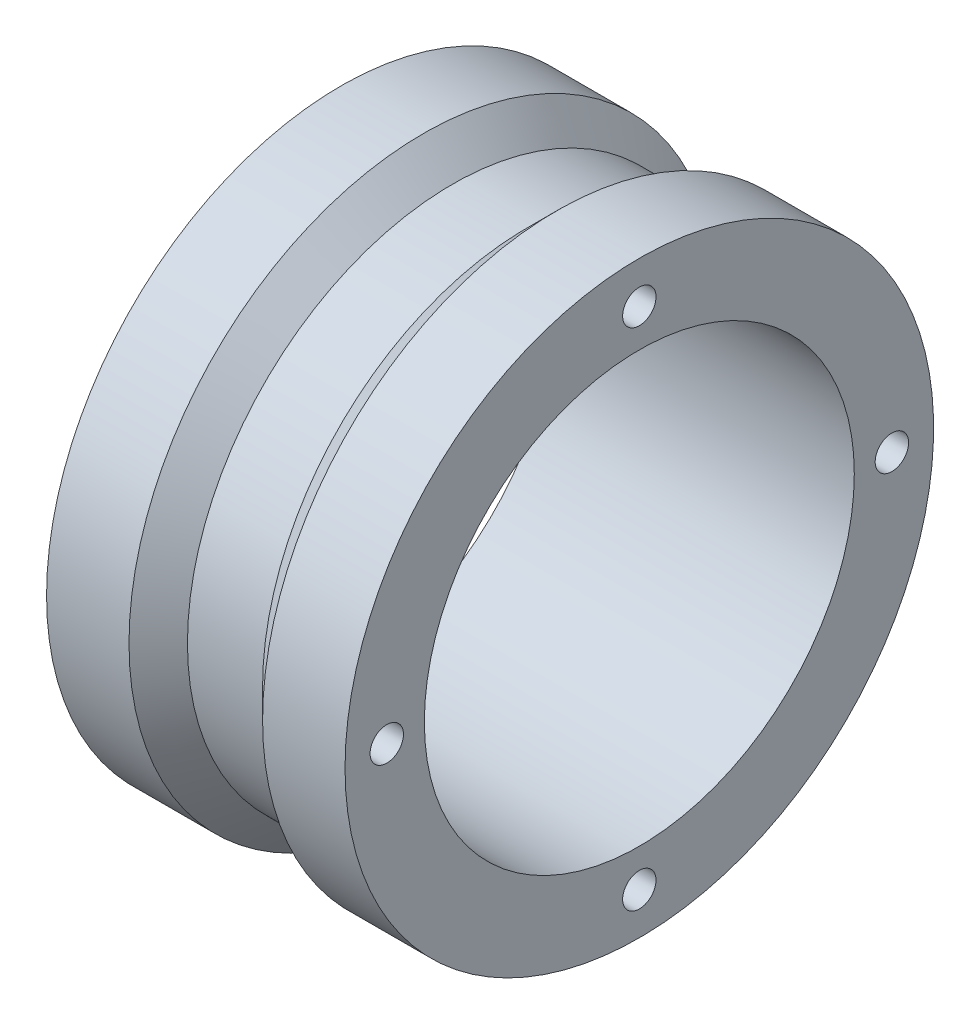
SolidWorks part; units mm, degrees
ref_plane "Front Plane" through (0, 0, 0) normal (0, 0, 1) x (1, 0, 0)
ref_plane "Top Plane" through (0, 0, 0) normal (0, 1, 0) x (1, 0, 0)
ref_plane "Right Plane" through (0, 0, 0) normal (1, 0, 0) x (0, 0, -1)
sketch "Sketch2" plane through (0, 0, 0) normal (0, 0, 1) x (1, 0, 0)
  line L0 (-86.7079, 0) -> (94.8794, 0) construction
  line L1 (-37.2254, 70.5) -> (-37.2254, 51.5)
  line L2 (-37.2254, 51.5) -> (34.2746, 51.5)
  line L3 (34.2746, 51.5) -> (34.2746, 70.5)
  line L4 (34.2746, 70.5) -> (14.5246, 70.5)
  line L6 (7.5246, 63.5) -> (-10.4754, 63.5)
  line L8 (-17.4754, 70.5) -> (-37.2254, 70.5)
  line L10 (-17.4754, 70.5) -> (-10.4754, 63.5)
  line L11 (14.5246, 70.5) -> (7.5246, 63.5)
  dimension "D1" = 71.5
  dimension "D2" = 18
  dimension "D3" = 70.5
  dimension "D4" = 51.5
  dimension "D5" = 70.5
  dimension "D7" = 7
revolve "Revolve1" add sketch "Sketch2" angle 360 about L0
sketch "Sketch4" plane through (-37.2254, 0, 0) normal (-1, 0, 0) x (0, 0, 1)
  circle A1 centre (0, -60.5) radius 4
  circle A2 centre (-60.5, 0) radius 4
  circle A3 centre (0, 60.5) radius 4
  circle A4 centre (60.5, 0) radius 4
  point P14 (0, 0)
  dimension "D2" = 8
  dimension "D3" = 4
extrude "Cut-Extrude1" cut sketch "Sketch4" against normal blind 13
sketch "Sketch5" plane through (34.2746, 0, 0) normal (1, 0, 0) x (0, 0, -1)
  circle A1 centre (0, -60.5) radius 4
  circle A2 centre (-60.5, 0) radius 4
  circle A3 centre (0, 60.5) radius 4
  circle A4 centre (60.5, 0) radius 4
  point P14 (0, 0)
  dimension "D2" = 8
  dimension "D3" = 4
extrude "Cut-Extrude2" cut sketch "Sketch5" against normal blind 13
